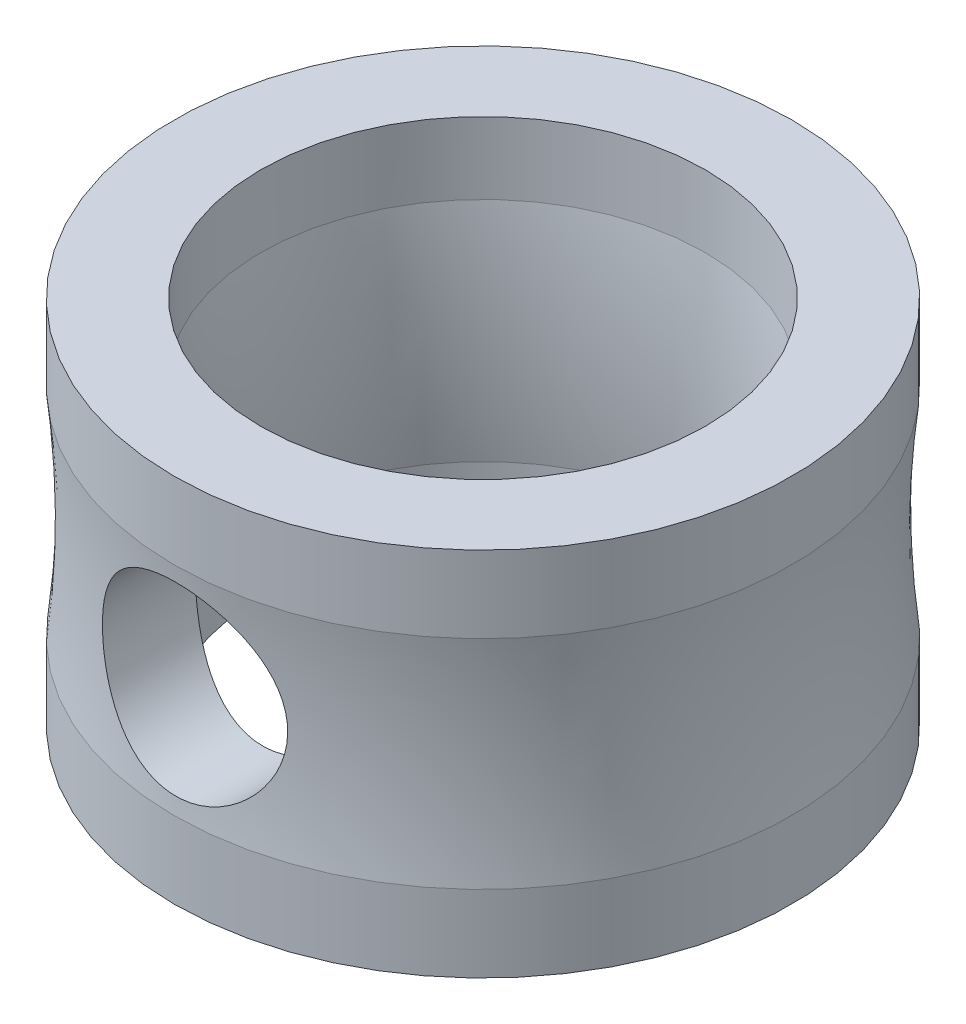
from build123d import *

# Parameters (mm, degrees)
SHELL1_T           = -70
SKETCH2_R          = 75
CUT_EXTRUDE1_DEPTH = 689


with BuildPart() as part:
    # Sketch1 → Revolve1 (revolve)
    with BuildSketch(Plane.XY, mode=Mode.PRIVATE) as revolve1_sk:
        with BuildLine():
            Line((0, 0), (0, 300))
            Line((0, 300), (250, 300))
            Line((250, 300), (250, 237.890484124))
            ThreePointArc((250, 237.890484124), (244.867735294, 150), (250, 62.109515876))
            Line((250, 62.109515876), (250, 0))
            Line((250, 0), (0, 0))
        make_face()
    revolve(revolve1_sk.sketch.rotate(Axis((0, 0, 0), (0, 1, 0)), 90), axis=Axis((0, 0, 0), (0, 1, 0)))

    # Shell1
    shell1_openings = [part.faces().sort_by_distance(p)[0] for p in [
        (0, 300, 0),
        (0, 0, 0),
    ]]
    offset(amount=SHELL1_T, openings=shell1_openings, kind=Kind.INTERSECTION)

    # Sketch2 → Cut-Extrude1 (cut)
    with BuildSketch(Plane.XY):
        with Locations(Location((0, 150, 0), (0, 0, 222.553028983))):
            Circle(SKETCH2_R)
    extrude(amount=CUT_EXTRUDE1_DEPTH, mode=Mode.SUBTRACT)


solid = part.part
